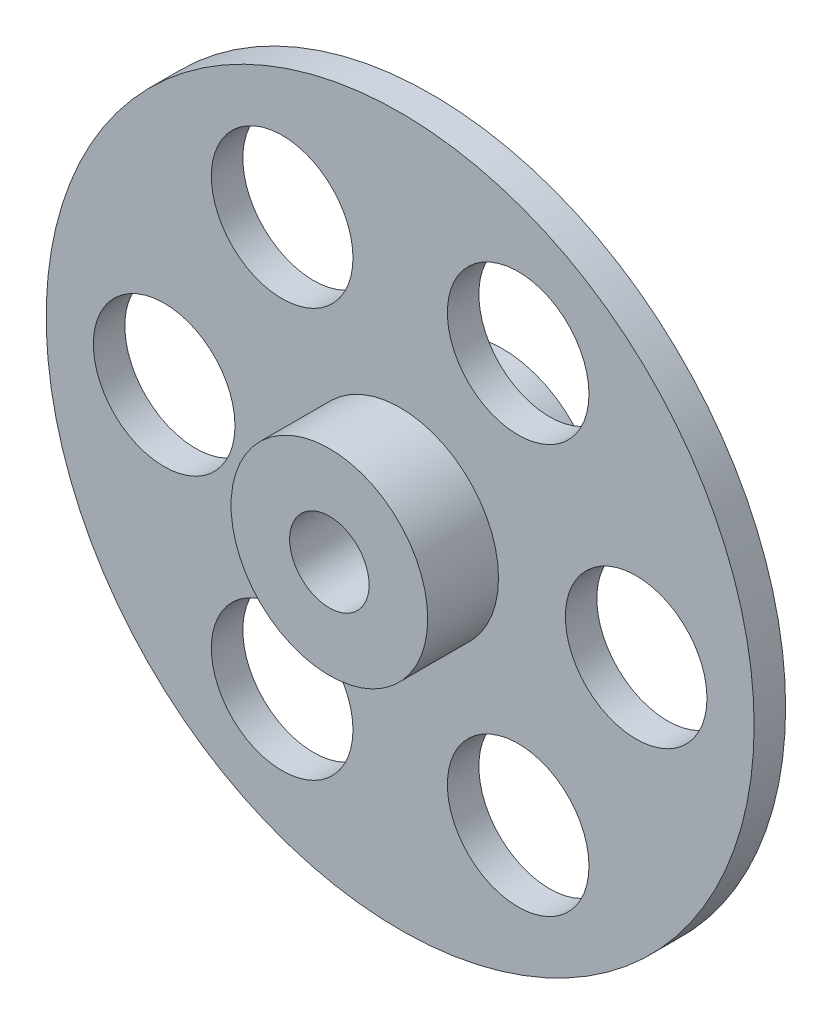
SolidWorks part; units mm, degrees
ref_plane "前视基准面" through (0, 0, 0) normal (0, 0, 1) x (1, 0, 0)
ref_plane "上视基准面" through (0, 0, 0) normal (0, 1, 0) x (1, 0, 0)
ref_plane "右视基准面" through (0, 0, 0) normal (1, 0, 0) x (0, 0, -1)
other "Configuration Table"
sketch "草图1" plane through (0, 0, 0) normal (0, 0, 1) x (1, 0, 0)
  circle A0 centre (0, 0) radius 90
  circle A1 centre (0, 0) radius 10.1
  point P0 (0, 0)
  dimension "D1" = 20.2
  dimension "D2" = 180
extrude "凸台-拉伸1" add sketch "草图1" against normal mid plane 8
sketch "草图2" plane through (0, 0, 0) normal (0, 0, 1) x (1, 0, 0)
  circle A0 centre (0, 0) radius 25
  circle A1 centre (0, 0) radius 10.1
  point P0 (0, 0)
  dimension "D1" = 20.2
  dimension "D2" = 50
extrude "凸台-拉伸2" add sketch "草图2" against normal mid plane 44
sketch "草图3" plane through (0, 0, 0) normal (0, 0, 1) x (1, 0, 0)
  circle A0 centre (60, 0) radius 18
  circle A1 centre (30, 51.9615) radius 18
  circle A2 centre (-30, 51.9615) radius 18
  circle A3 centre (-60, 0) radius 18
  circle A4 centre (-30, -51.9615) radius 18
  circle A5 centre (30, -51.9615) radius 18
  point P0 (0, 0)
  dimension "D1" = 36
  dimension "D2" = 36
  dimension "D3" = 36
  dimension "D4" = 36
  dimension "D5" = 36
  dimension "D6" = 36
  dimension "D7" = 30
  dimension "D8" = 60
  dimension "D9" = 90
  dimension "D10" = 120
  dimension "D11" = 51.9615
  dimension "D12" = 103.923
extrude "切除-拉伸1" cut sketch "草图3" against normal mid plane 60
